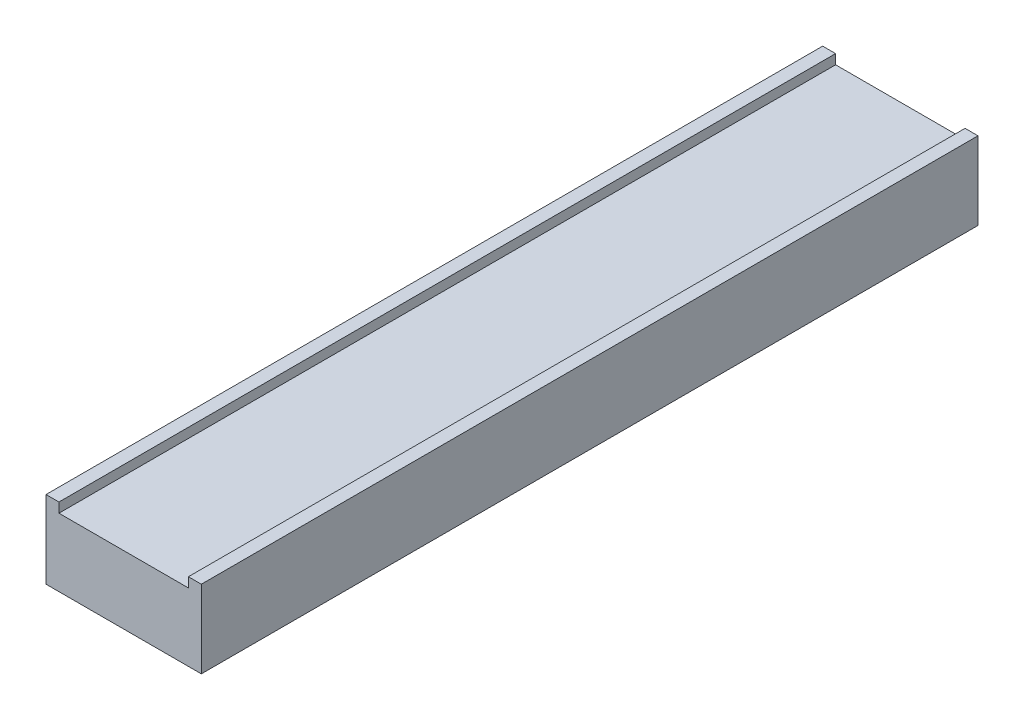
from build123d import *

# Parameters (mm, degrees)
SKETCH_1_W          = 12
SKETCH_1_H          = 60
EXTRUDE_1_DEPTH     = 6
SKETCH_2_W          = 10
SKETCH_2_H          = 60
CUT_EXTRUDE_1_DEPTH = 0.75


with BuildPart() as part:
    # 草图1 → 凸台-拉伸1 (new body)
    with BuildSketch(Plane(origin=(0, 0, 0), x_dir=(1, 0, 0), z_dir=(0, 1, 0))):
        Rectangle(SKETCH_1_W, SKETCH_1_H)
    extrude(amount=EXTRUDE_1_DEPTH)

    # 草图2 → 切除-拉伸1 (cut)
    with BuildSketch(Plane(origin=(0, 6, 0), x_dir=(1, 0, 0), z_dir=(0, 1, 0))):
        Rectangle(SKETCH_2_W, SKETCH_2_H)
    extrude(amount=-CUT_EXTRUDE_1_DEPTH, mode=Mode.SUBTRACT)


solid = part.part
